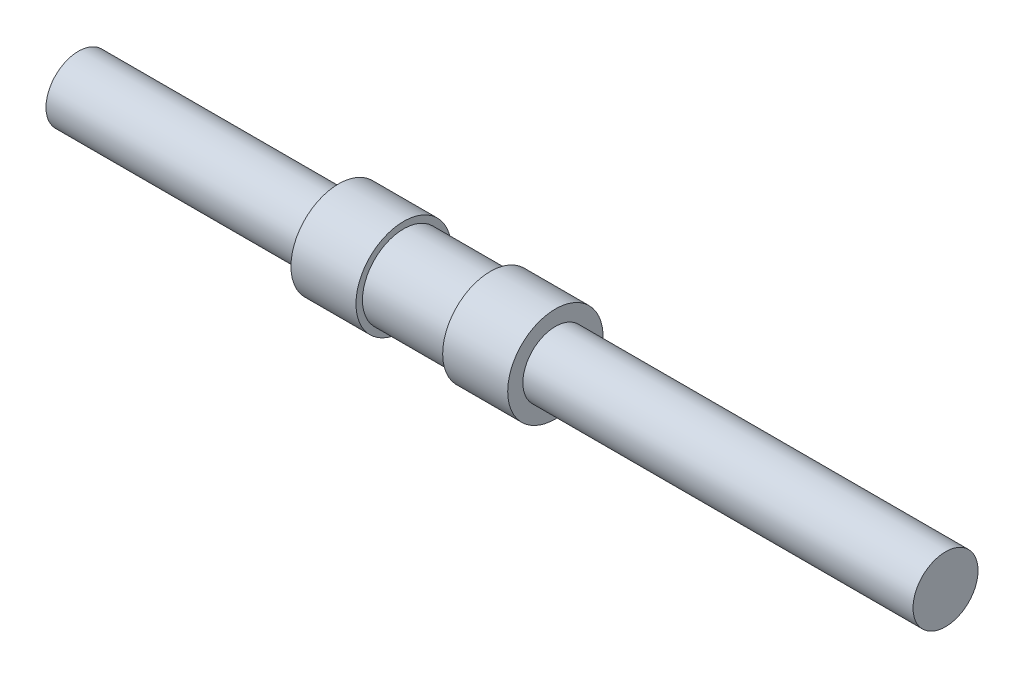
SolidWorks part; units mm, degrees
material "6061"
ref_plane "前视基准面" through (0, 0, 0) normal (0, 0, 1) x (1, 0, 0)
ref_plane "上视基准面" through (0, 0, 0) normal (0, 1, 0) x (1, 0, 0)
ref_plane "右视基准面" through (0, 0, 0) normal (1, 0, 0) x (0, 0, -1)
sketch "草图1" plane through (0, 0, 0) normal (0, 0, 1) x (1, 0, 0)
  line L0 (0, 0) -> (400, 0) construction
  line L1 (0, 0) -> (0, 15)
  line L2 (0, 15) -> (120, 15)
  line L3 (120, 15) -> (120, 22)
  line L4 (120, 22) -> (150, 22)
  line L5 (150, 22) -> (150, 19)
  line L6 (150, 19) -> (190, 19)
  line L7 (190, 19) -> (190, 22)
  line L8 (190, 22) -> (220, 22)
  line L9 (220, 22) -> (220, 15)
  line L10 (220, 15) -> (400, 15)
  line L11 (400, 15) -> (400, 0)
  line L12 (0, 0) -> (400, 0)
  dimension "D1" = 30
  dimension "D2" = 44
  dimension "D3" = 3
  dimension "D4" = 400
  dimension "D5" = 120
  dimension "D6" = 100
  dimension "D7" = 30
revolve "旋转1" add sketch "草图1" angle 360 about L0
sketch "草图2" plane through (0, 0, 0) normal (-1, 0, 0) x (0, 0, 1)
  circle A0 centre (0, 0) radius 13.5
  dimension "D1" = 27
extrude "螺纹孔M28*1.0" cut sketch "草图2" against normal blind 300
cosmetic thread "装饰螺纹线1" parameters "D1"=15, "D2"=28
